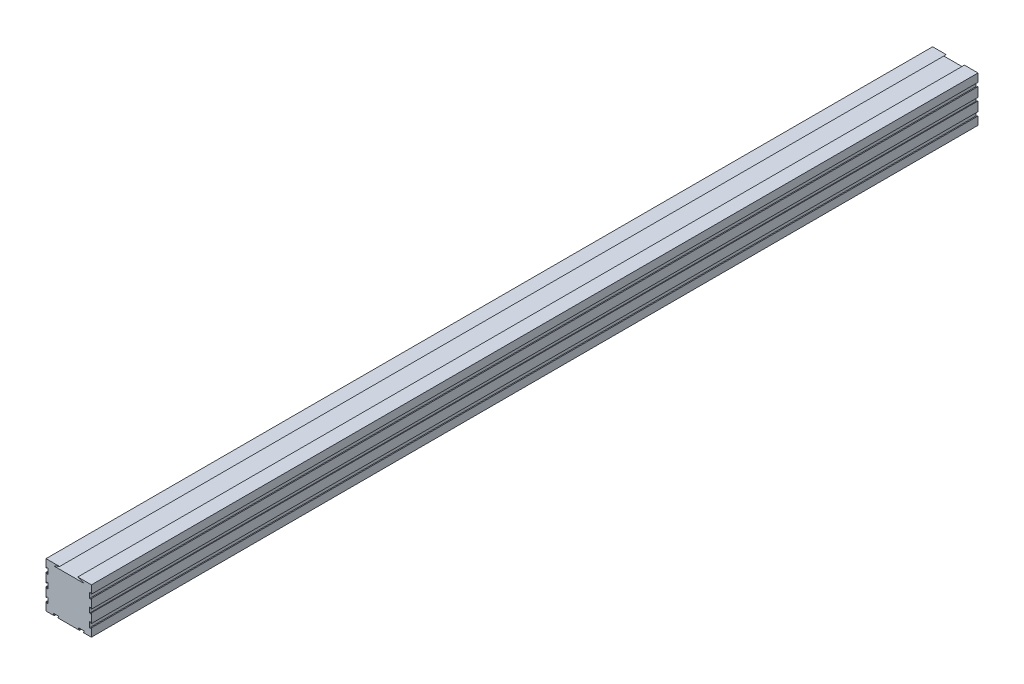
SolidWorks part; units mm, degrees
ref_plane "前视基准面" through (0, 0, 0) normal (0, 0, 1) x (1, 0, 0)
ref_plane "上视基准面" through (0, 0, 0) normal (0, 1, 0) x (1, 0, 0)
ref_plane "右视基准面" through (0, 0, 0) normal (1, 0, 0) x (0, 0, -1)
sketch "草图1" plane through (0, 0, 0) normal (0, 0, 1) x (1, 0, 0)
  line L1 (-37.5, 37.5) -> (37.5, 37.5)
  line L2 (-37.5, 37.5) -> (-37.5, -37.5)
  line L3 (-37.5, -37.5) -> (37.5, -37.5)
  line L4 (37.5, 37.5) -> (37.5, -37.5)
  line L5 (-37.5, 37.5) -> (37.5, -37.5) construction
  line L6 (-37.5, -37.5) -> (37.5, 37.5) construction
  point P0 (0, 0)
  dimension "D1" = 75
  dimension "D2" = 75
extrude "凸台-拉伸1" add sketch "草图1" along normal mid plane 1465 contours L1 L4 L3 L2
sketch "草图2" plane through (0, 0, 0) normal (0, 0, 1) x (1, 0, 0)
  line L0 (-37.5, -37.5) -> (37.5, -37.5) construction
  line L1 (-17.9, -36.8) -> (-16.55, -36.8)
  line L2 (-24.1, -36.8) -> (-24.1, -37.5)
  line L3 (-24.1, -37.5) -> (-17.9, -37.5)
  line L4 (-17.9, -36.8) -> (-17.9, -37.5)
  line L5 (-21, -38.432) -> (-21, -32.3332) construction
  line L6 (-25.45, -34.5) -> (-16.55, -34.5)
  line L7 (-25.45, -34.5) -> (-25.45, -36.8)
  line L8 (-25.45, -36.8) -> (-24.1, -36.8)
  line L9 (-16.55, -34.5) -> (-16.55, -36.8)
  line L10 (0, -20.0698) -> (0, -49.6644) construction
  line L11 (21, -38.432) -> (21, -32.3332) construction
  line L12 (16.55, -34.5) -> (16.55, -36.8)
  line L13 (25.45, -36.8) -> (24.1, -36.8)
  line L14 (25.45, -34.5) -> (25.45, -36.8)
  line L15 (25.45, -34.5) -> (16.55, -34.5)
  line L16 (17.9, -36.8) -> (17.9, -37.5)
  line L17 (24.1, -37.5) -> (17.9, -37.5)
  line L18 (24.1, -36.8) -> (24.1, -37.5)
  line L19 (17.9, -36.8) -> (16.55, -36.8)
  dimension "D1" = 6.2
  dimension "D2" = 8.9
  dimension "D3" = 0.7
  dimension "D4" = 2.3
  dimension "D5" = 3.1
  dimension "D6" = 4.45
  dimension "D7" = 21
extrude "切除-拉伸1" cut sketch "草图2" against normal mid plane 1465
sketch "草图3" plane through (0, 0, 732.5) normal (0, 0, 1) x (1, 0, 0)
  line L0 (37.5, 37.5) -> (37.5, -37.5) construction
  line L1 (37.5, 2.6) -> (36.8, 2.6)
  line L2 (37.5, 2.6) -> (37.5, -2.6)
  line L3 (37.5, -2.6) -> (36.8, -2.6)
  line L4 (36.8, -2.6) -> (36.8, -4.45)
  line L5 (0, 0) -> (42.093, 0) construction
  line L6 (34.5, 4.45) -> (36.8, 4.45)
  line L7 (34.5, 4.45) -> (34.5, -4.45)
  line L8 (34.5, -4.45) -> (36.8, -4.45)
  line L9 (36.8, 4.45) -> (36.8, 2.6)
  line L10 (39.5858, -21) -> (29.5778, -21) construction
  line L11 (37.5, -17.9) -> (36.8, -17.9)
  line L12 (37.5, -17.9) -> (37.5, -24.1)
  line L13 (37.5, -24.1) -> (36.8, -24.1)
  line L14 (39.5858, 21) -> (29.5778, 21) construction
  line L15 (34.5, -16.55) -> (36.8, -16.55)
  line L16 (34.5, -16.55) -> (34.5, -25.45)
  line L17 (34.5, -25.45) -> (36.8, -25.45)
  line L18 (36.8, -16.55) -> (36.8, -17.9)
  line L19 (36.8, -24.1) -> (36.8, -25.45)
  line L20 (36.8, 24.1) -> (36.8, 25.45)
  line L21 (36.8, 16.55) -> (36.8, 17.9)
  line L22 (34.5, 25.45) -> (36.8, 25.45)
  line L23 (34.5, 16.55) -> (34.5, 25.45)
  line L24 (34.5, 16.55) -> (36.8, 16.55)
  line L25 (37.5, 24.1) -> (36.8, 24.1)
  line L26 (37.5, 17.9) -> (37.5, 24.1)
  line L27 (37.5, 17.9) -> (36.8, 17.9)
  line L28 (0, 28.4328) -> (0, -27.557) construction
  dimension "D1" = 5.2
  dimension "D2" = 2.6
  dimension "D3" = 8.9
  dimension "D4" = 4.45
  dimension "D5" = 0.7
  dimension "D6" = 2.3
  dimension "D7" = 6.2
  dimension "D8" = 8.9
  dimension "D9" = 3.1
  dimension "D10" = 4.45
  dimension "D11" = 0.7
  dimension "D12" = 2.3
  dimension "D13" = 21
extrude "切除-拉伸2" cut sketch "草图3" against normal blind 1465
mirror "镜向1" about plane through (0, 0, 0) normal (1, 0, 0) of "切除-拉伸2"
sketch "草图4" plane through (0, 0, 732.5) normal (0, 0, 1) x (1, 0, 0)
  line L0 (-15, 37.5) -> (-25, 33.5)
  line L1 (-37.5, 37.5) -> (37.5, 37.5) construction
  line L2 (-25, 33.5) -> (25, 33.5)
  line L3 (25, 33.5) -> (15, 37.5)
  dimension "D1" = 50
  dimension "D2" = 25
  dimension "D3" = 30
  dimension "D4" = 15
  dimension "D5" = 4
extrude "切除-拉伸3" cut sketch "草图4" against normal through all and the other way through all
